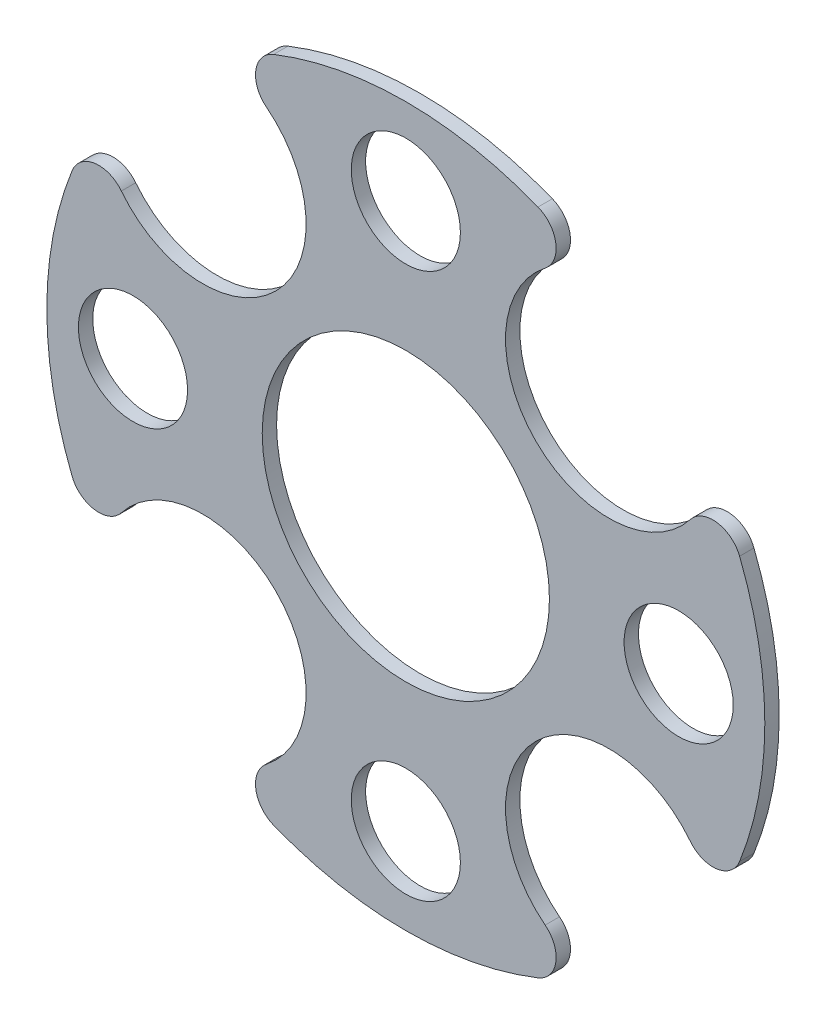
SolidWorks part; units mm, degrees
material "H62"
ref_plane "Front Plane" through (0, 0, 0) normal (0, 0, 1) x (1, 0, 0)
ref_plane "Top Plane" through (0, 0, 0) normal (0, 1, 0) x (1, 0, 0)
ref_plane "Right Plane" through (0, 0, 0) normal (1, 0, 0) x (0, 0, -1)
sketch "Sketch1" plane through (0, 0, 0) normal (0, 0, 1) x (1, 0, 0)
  line L0 (0, 0) -> (0, 31.2951) construction
  line L1 (0, 0) -> (40.2652, 0) construction
  line L2 (7.0711, 7.0711) -> (-7.0711, -7.0711) construction
  line L3 (-7.0711, 7.0711) -> (7.0711, -7.0711) construction
  arc A0 (-11.6219, 4.6024) -> (-11.6219, -4.6024) centre (0, 0) ccw
  arc A1 (-4.8509, 9.9049) -> (-9.9049, 4.8509) centre (-7.0711, 7.0711) cw
  arc A2 (4.8509, 9.9049) -> (9.9049, 4.8509) centre (7.0711, 7.0711) ccw
  arc A3 (4.8509, -9.9049) -> (9.9049, -4.8509) centre (7.0711, -7.0711) cw
  arc A4 (-4.8509, -9.9049) -> (-9.9049, -4.8509) centre (-7.0711, -7.0711) ccw
  arc A5 (-4.6024, -11.6219) -> (4.6024, -11.6219) centre (0, 0) ccw
  arc A6 (11.6219, -4.6024) -> (11.6219, 4.6024) centre (0, 0) ccw
  arc A7 (4.6024, 11.6219) -> (-4.6024, 11.6219) centre (0, 0) ccw
  arc A8 (9.9049, -4.8509) -> (11.6219, -4.6024) centre (10.6921, -4.2342) ccw
  arc A9 (4.8509, -9.9049) -> (4.6024, -11.6219) centre (4.2342, -10.6921) cw
  arc A10 (-4.8509, -9.9049) -> (-4.6024, -11.6219) centre (-4.2342, -10.6921) ccw
  arc A11 (-9.9049, -4.8509) -> (-11.6219, -4.6024) centre (-10.6921, -4.2342) cw
  arc A12 (4.8509, 9.9049) -> (4.6024, 11.6219) centre (4.2342, 10.6921) ccw
  arc A13 (-4.8509, 9.9049) -> (-4.6024, 11.6219) centre (-4.2342, 10.6921) cw
  arc A14 (9.9049, 4.8509) -> (11.6219, 4.6024) centre (10.6921, 4.2342) cw
  arc A15 (-9.9049, 4.8509) -> (-11.6219, 4.6024) centre (-10.6921, 4.2342) ccw
  circle A16 centre (0, 0) radius 10 construction
  circle A17 centre (0, 0) radius 5
  circle A18 centre (0, 9.5) radius 1.9
  circle A19 centre (0, 0) radius 9.5 construction
  circle A20 centre (9.5, 0) radius 1.9
  circle A21 centre (0, -9.5) radius 1.9
  circle A22 centre (-9.5, 0) radius 1.9
  dimension "D1" = 25
  dimension "D2" = 7.2
  dimension "D3" = 1
  dimension "D4" = 20
  dimension "D6" = 10
  dimension "D7" = 19
  dimension "D8" = 3.8
  dimension "D5" = 45
extrude "Boss-Extrude1" add sketch "Sketch1" along normal blind 0.5
